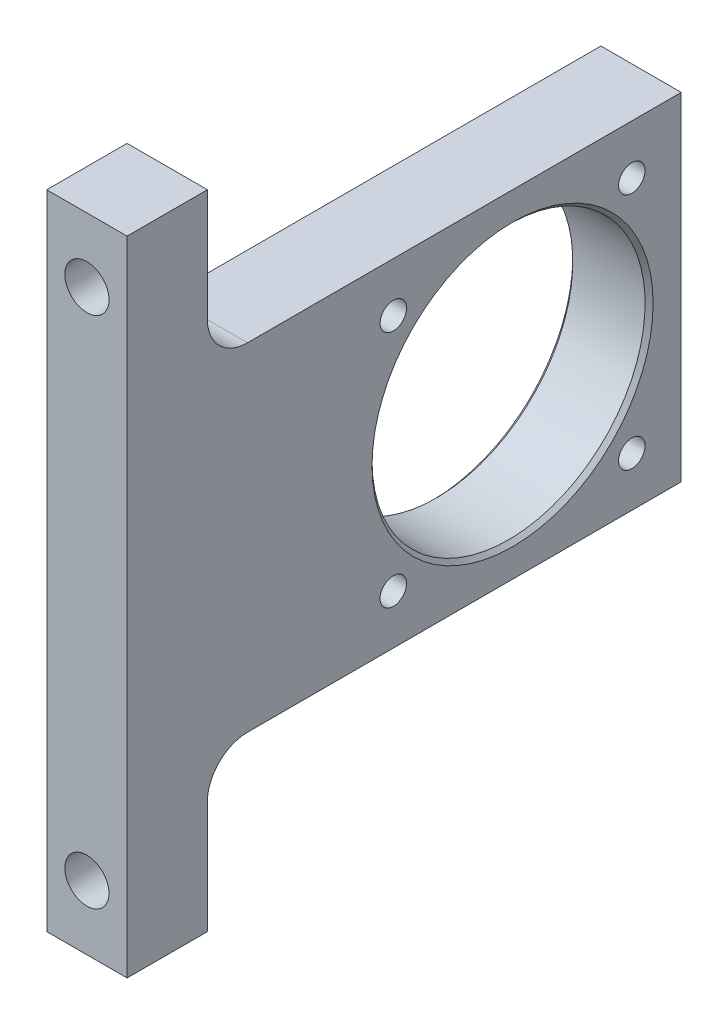
from build123d import *

# Parameters (mm, degrees)
BOSS_EXTRUDE1_DEPTH        = 10
SKETCH2_R                  = 17
CUT_EXTRUDE1_DEPTH         = 81.380345856
F_5_5_5_5_DIAMETER_HOLE1_D = 5.5
M4_TAPPED_HOLE1_D          = 3.3
FILLET1_R                  = 5
CHAMFER1_SIZE              = 0.5


with BuildPart() as part:
    # Sketch1 → Boss-Extrude1 (new body)
    with BuildSketch(Plane(origin=(0, 0, 0), x_dir=(0, 0, -1), z_dir=(1, 0, 0))):
        Polygon((0, -40), (0, 40), (10, 40), (10, 21), (69, 21), (69, -21), (10, -21), (10, -40), align=None)
    extrude(amount=BOSS_EXTRUDE1_DEPTH)

    # Sketch2 → Cut-Extrude1 (cut, through all)
    with BuildSketch(Plane(origin=(10, 0, 0), x_dir=(0, 0, -1), z_dir=(1, 0, 0))):
        with Locations((48, 0)):
            Circle(SKETCH2_R)
    extrude(amount=-CUT_EXTRUDE1_DEPTH, mode=Mode.SUBTRACT)

    # Ø5.5 (5.5) Diameter Hole1 (through all)
    with Locations(Plane.XY):
        with Locations((5, 32), (5, -32)):
            Hole(F_5_5_5_5_DIAMETER_HOLE1_D / 2)

    # M4 Tapped Hole1 (through all)
    with Locations(Plane(origin=(10, 0, 0), x_dir=(0, 0, -1), z_dir=(1, 0, 0))):
        with Locations((33.150757595, 14.849242405), (62.849242405, 14.849242405), (62.849242405, -14.849242405), (33.150757595, -14.849242405)):
            Hole(M4_TAPPED_HOLE1_D / 2)

    # Fillet1
    fillet1_edges = [part.edges().sort_by_distance(p)[0] for p in [
        (5, 21, -10),
        (5, -21, -10),
    ]]
    fillet(fillet1_edges, radius=FILLET1_R)

    # Chamfer1
    chamfer1_edges = [part.edges().sort_by_distance(p)[0] for p in [
        (0, 0, -31),
        (10, 0, -31),
    ]]
    chamfer(chamfer1_edges, length=CHAMFER1_SIZE)


solid = part.part
